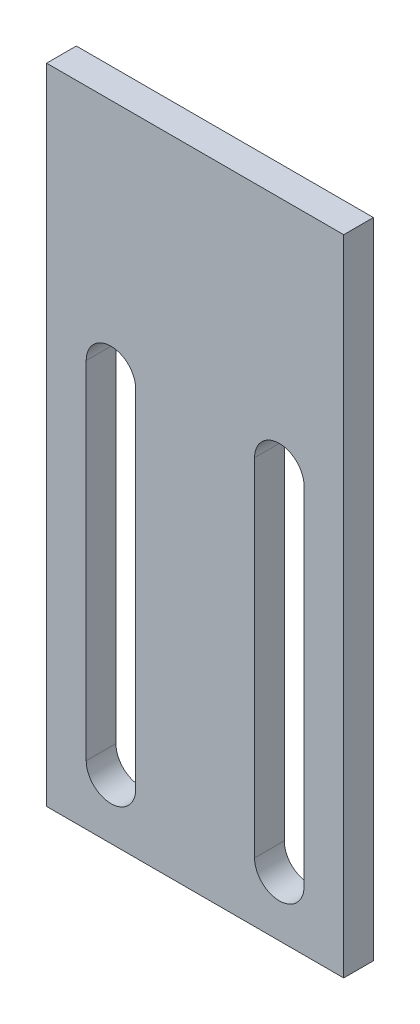
from build123d import *

# Parameters (mm, degrees)
SKETCH_1_W          = 30
SKETCH_1_H          = 65
EXTRUDE_1_DEPTH     = 3
CUT_EXTRUDE_1_REACH = 37.92


with BuildPart() as part:
    # 草图1 → 凸台-拉伸1 (new body)
    with BuildSketch(Plane.XY):
        Rectangle(SKETCH_1_W, SKETCH_1_H)
    extrude(amount=EXTRUDE_1_DEPTH)

    # 草图2 → 切除-拉伸1 (cut, up to next)
    with BuildSketch(Plane.XY.offset(3), mode=Mode.PRIVATE) as cut_extrude_1_sk1:
        with BuildLine():
            Line((-11, -26.5), (-11, 8.5))
            ThreePointArc((-11, 8.5), (-8.5, 11), (-6, 8.5))
            Line((-6, 8.5), (-6, -26.5))
            ThreePointArc((-6, -26.5), (-8.5, -29), (-11, -26.5))
        make_face()
    cut_extrude_1_tool1 = extrude(cut_extrude_1_sk1.sketch, amount=-CUT_EXTRUDE_1_REACH, mode=Mode.PRIVATE) & part.part
    cut_extrude_1 = cut_extrude_1_tool1.solids().sort_by_distance((-8.5, -9, 3))[0]
    add(cut_extrude_1, mode=Mode.SUBTRACT)

    # 镜向1: 切除-拉伸1 across plane
    add(cut_extrude_1.mirror(Plane(origin=(0, 0, 0), x_dir=(0, 0, 1), z_dir=(1, 0, 0))), mode=Mode.SUBTRACT)


solid = part.part
